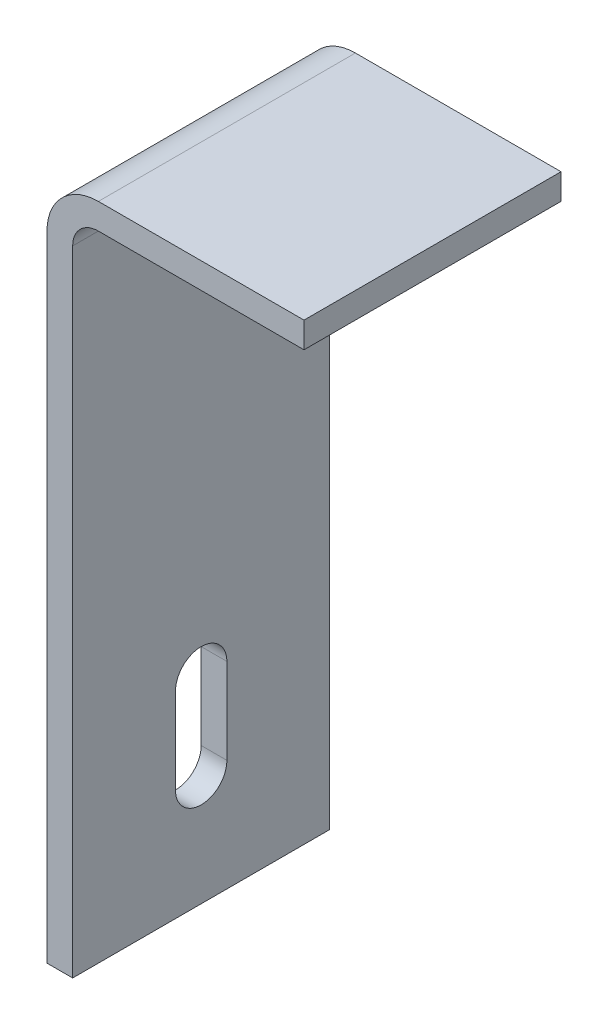
SolidWorks part; units mm, degrees
material "Plain Carbon Steel"
ref_plane "Front Plane" through (0, 0, 0) normal (0, 0, 1) x (1, 0, 0)
ref_plane "Top Plane" through (0, 0, 0) normal (0, 1, 0) x (1, 0, 0)
ref_plane "Right Plane" through (0, 0, 0) normal (1, 0, 0) x (0, 0, -1)
sketch "Sketch1" plane through (0, 0, 0) normal (0, 0, 1) x (1, 0, 0)
  line L0 (6, 0) -> (30, 0)
  line L1 (0, -6) -> (0, -80)
  arc A0 (6, 0) -> (0, -6) centre (6, -6) ccw
  point P6 (0, 0)
  dimension "D3" = 6
  dimension "D1" = 30
  dimension "D2" = 80
extrude "Extrude-Thin1" add sketch "Sketch1" along normal blind 30 thin
sketch "Sketch2" plane through (0, 0, 0) normal (-1, 0, 0) x (0, 0, 1)
  line L0 (15, -57) -> (15, -67) construction
  line L1 (18, -57) -> (18, -67)
  line L2 (12, -57) -> (12, -67)
  line L4 (30, 0) -> (0, 0) construction
  line L5 (30, -6) -> (30, -80) construction
  arc A0 (18, -57) -> (12, -57) centre (15, -57) ccw
  arc A1 (12, -67) -> (18, -67) centre (15, -67) ccw
  point P2 (15, -62)
  dimension "D3" = 3
  dimension "D1" = 62
  dimension "D2" = 10
  dimension "D4" = 15
extrude "Cut-Extrude1" cut sketch "Sketch2" against normal blind 3
